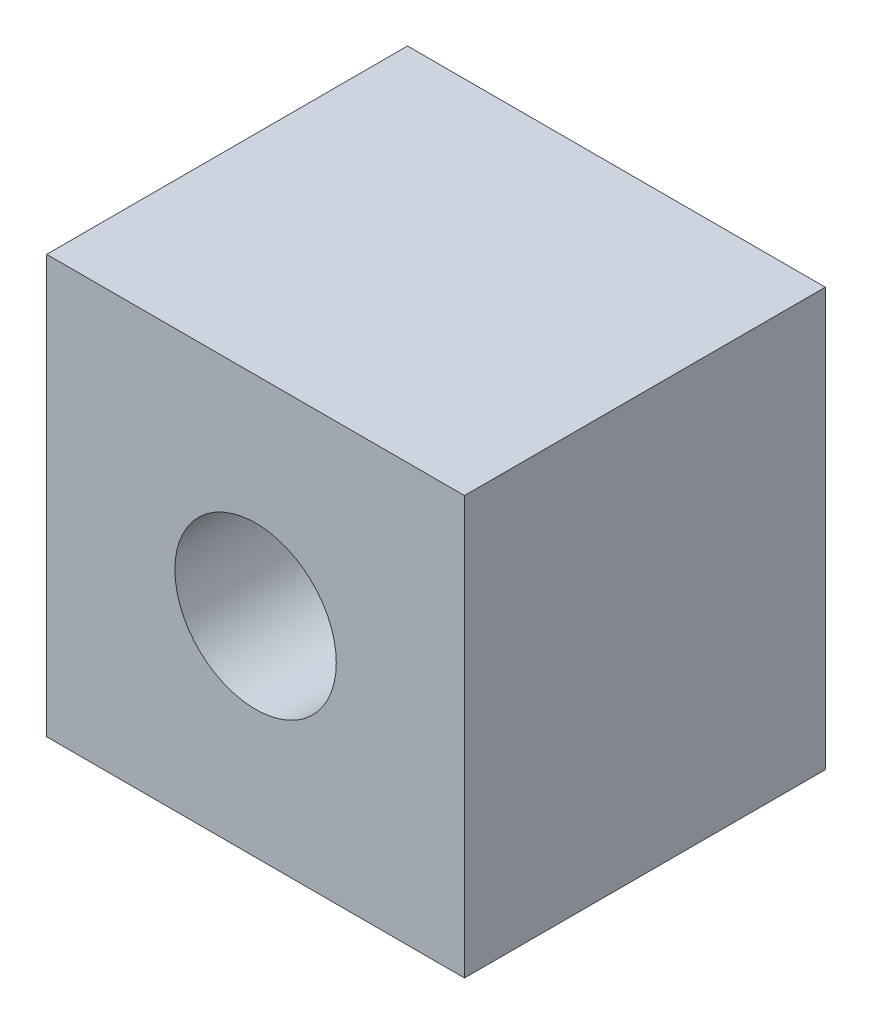
SolidWorks part; units mm, degrees
material "SS400B"
ref_plane "Front Plane" through (0, 0, 0) normal (0, 0, 1) x (1, 0, 0)
ref_plane "Top Plane" through (0, 0, 0) normal (0, 1, 0) x (1, 0, 0)
ref_plane "Right Plane" through (0, 0, 0) normal (1, 0, 0) x (0, 0, -1)
sketch "Sketch1" plane through (0, 0, 0) normal (0, 0, 1) x (1, 0, 0)
  line L0 (855.7723, 986.1628) -> (877.7723, 986.1628)
  line L1 (877.7723, 986.1628) -> (877.7723, 964.1628)
  line L2 (877.7723, 964.1628) -> (855.7723, 964.1628)
  line L3 (855.7723, 964.1628) -> (855.7723, 986.1628)
  circle A1 centre (866.7723, 975.1628) radius 4
  dimension "D1" = 22
  dimension "D3" = 8
  dimension "D5" = 11
  dimension "D2" = 22
  dimension "D4" = 11
extrude "Boss-Extrude1" add sketch "Sketch1" along normal blind 19
hole_wizard "M10 Tapped Hole2" positions "3DSketch1" profile "Sketch2" tap size "M10" standard "GB"
sketch3d "3DSketch1"
  line L0 (866.7723, 975.1628, 19) -> (866.7723, 975.1628, 0) construction
  point P0 (866.7723, 975.1628, 19)
sketch "Sketch2" plane through (866.7723, 975.1628, 19) normal (1, 0, 0) x (0, -1, 0)
  line L0 (0, 0) -> (0, 30.0537)
  line L1 (0, 30.0537) -> (4.25, 27.5)
  line L2 (4.25, 27.5) -> (4.25, 0)
  line L5 (4.25, 0) -> (0, 0)
  line L10 (0, 30.0537) -> (-4.25, 27.5) construction
  line L11 (0, -6.35) -> (0, 107.95) construction
  dimension "螺纹孔钻头直径" = 8.5
  dimension "螺纹孔钻头深度" = 27.5
  dimension "导头角度" = 118
cosmetic thread "Cosmetic-Thread1" parameters "D1"=19, "D2"=10
